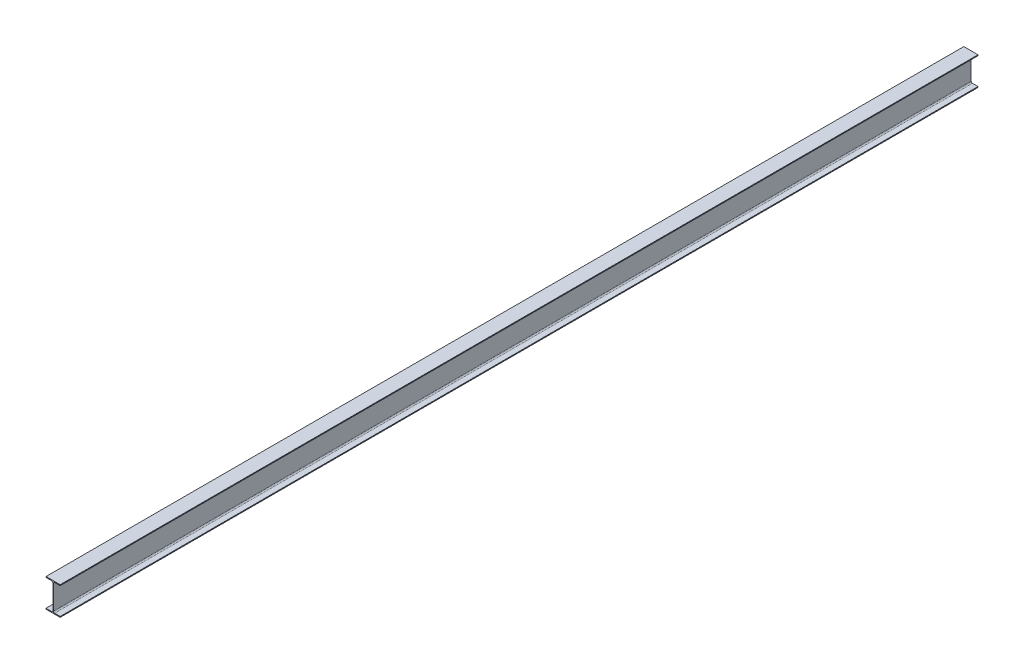
SolidWorks part; units mm, degrees
ref_plane "Front Plane" through (0, 0, 0) normal (0, 0, 1) x (1, 0, 0)
ref_plane "Top Plane" through (0, 0, 0) normal (0, 1, 0) x (1, 0, 0)
ref_plane "Right Plane" through (0, 0, 0) normal (1, 0, 0) x (0, 0, -1)
other "Configuration Table"
sketch "Sketch1" plane through (0, 0, 0) normal (0, 0, 1) x (1, 0, 0)
  line L0 (0, 0) -> (0, 300) construction
  line L1 (75, 0) -> (-75, 0)
  line L2 (-75, 0) -> (-75, 9)
  line L3 (-75, 9) -> (-16.25, 9)
  line L4 (3.25, 22) -> (3.25, 278)
  line L6 (-75, 291) -> (-75, 300)
  line L7 (-75, 300) -> (75, 300)
  line L8 (-3.25, 22) -> (-3.25, 278)
  line L9 (75, 291) -> (75, 300)
  line L10 (16.25, 291) -> (75, 291)
  line L11 (75, 9) -> (16.25, 9)
  line L12 (75, 0) -> (75, 9)
  line L13 (-16.25, 291) -> (-75, 291)
  arc A0 (16.25, 9) -> (3.25, 22) centre (16.25, 22) cw
  arc A1 (-3.25, 22) -> (-16.25, 9) centre (-16.25, 22) cw
  arc A2 (3.25, 278) -> (16.25, 291) centre (16.25, 278) cw
  arc A3 (-3.25, 278) -> (-16.25, 291) centre (-16.25, 278) ccw
  point P18 (3.25, 9)
  point P21 (-3.25, 9)
  point P24 (3.25, 291)
  point P27 (-3.25, 291)
  dimension "D6" = 13
  dimension "D1" = 300
  dimension "D2" = 150
  dimension "D3" = 6.5
  dimension "D4" = 9
  dimension "D5" = 9
extrude "Boss-Extrude1" add sketch "Sketch1" along normal blind 9710
